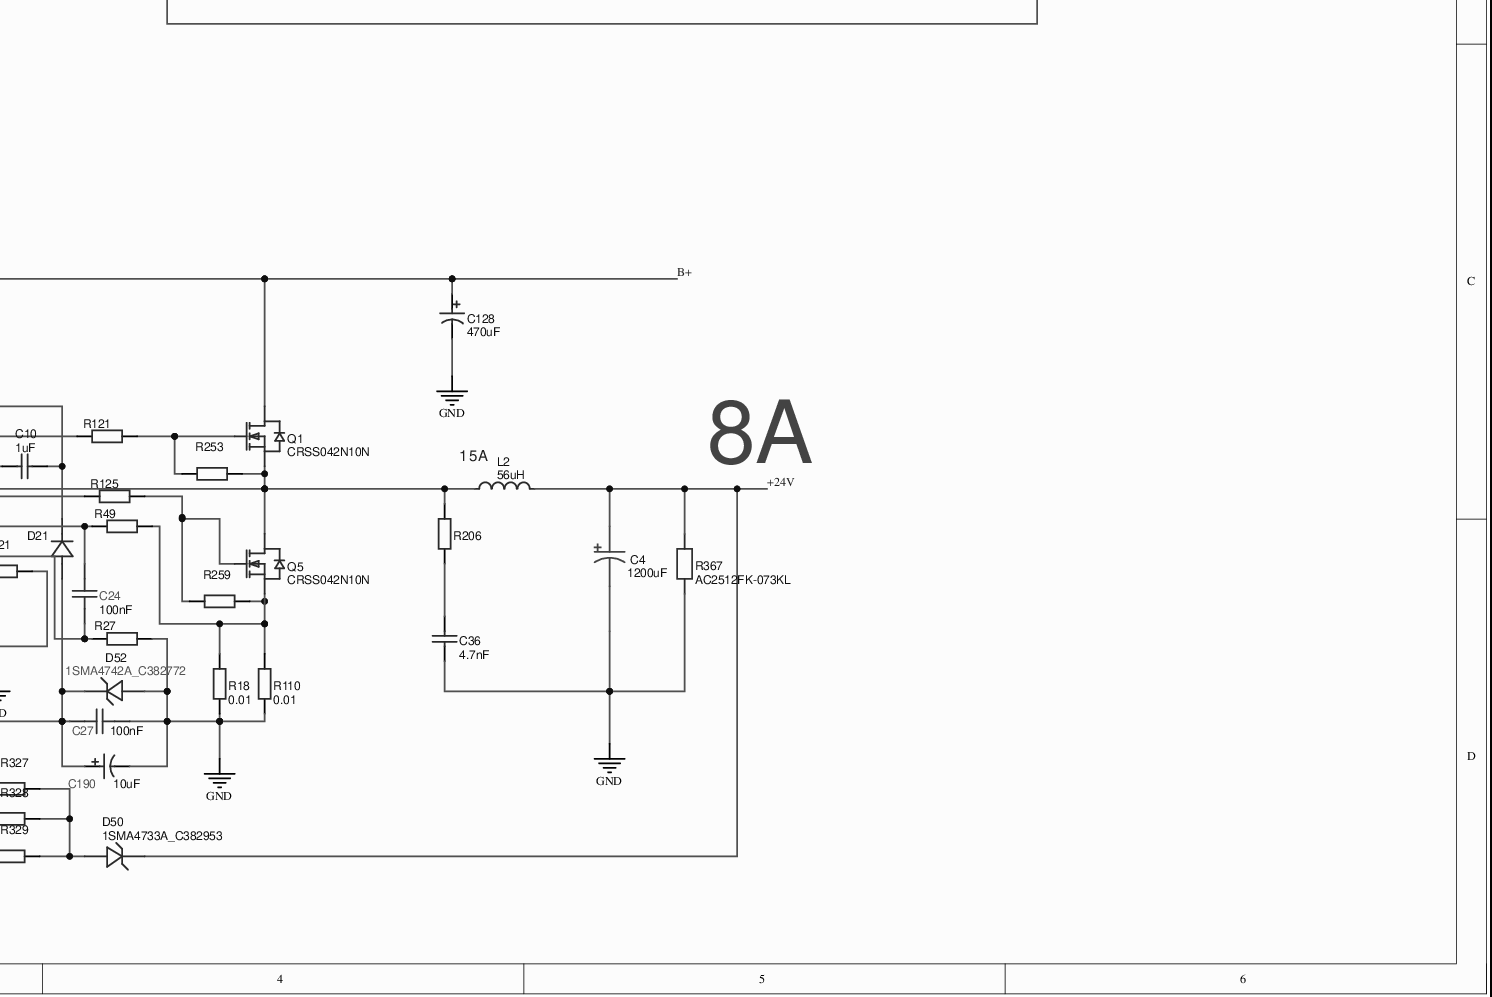
[diagram p0: MISC84402-12.SchDoc, bottom right]
# Altium project MISC84402-4.PrjPcb (part 5 of 7)
## Sheet MISC84402-12.SchDoc (continued)
### Library data of the parts (continued)
R34 = (no symbol name): BOM_Manufacturer: UniOhm; BOM_Manufacturer Part: 0603WAF7501T5E; nameAlias: Resistance; Resistance (Ohms): 7.5K; BOM_Supplier: LCSC; BOM_Supplier Part: C23234; BOM_JLCPCB Part Class: Basic Part; spicePre: R; spiceSymbolName: 0603WAF7501T5E
R48 R362 = (no symbol name): BOM_Manufacturer: UniOhm; BOM_Manufacturer Part: 0603WAF330JT5E; nameAlias: Resistance; Resistance (Ohms): 33; BOM_Supplier: LCSC; BOM_Supplier Part: C23140; BOM_JLCPCB Part Class: Basic Part; spicePre: R; spiceSymbolName: 0603WAF330JT5E
R51 R73 R291 R296 R302 R314 = 2K: BOM_Manufacturer: UniOhm; BOM_Manufacturer Part: 0603WAF2001T5E; nameAlias: Resistance (Ohms); BOM_Supplier: LCSC; BOM_Supplier Part: C22975; BOM_JLCPCB Part Class: Basic Part; spicePre: R; spiceSymbolName: 0603WAF2001T5E
R74 R101 R121 R125 = (no symbol name): BOM_Manufacturer: UniOhm; BOM_Manufacturer Part: 0805W8F220KT5E; nameAlias: Resistance; Resistance (Ohms): 2.2; BOM_Supplier: LCSC; BOM_Supplier Part: C17521; BOM_JLCPCB Part Class: Basic Part; spicePre: R; spiceSymbolName: 0805W8F220KT5E
R75 = (no symbol name): BOM_Manufacturer: UniOhm; BOM_Manufacturer Part: 0603WAF1003T5E; nameAlias: Resistance; Resistance (Ohms): 100K; BOM_Supplier: LCSC; BOM_Supplier Part: C25803; BOM_JLCPCB Part Class: Basic Part; spicePre: R; spiceSymbolName: 0603WAF1003T5E
R104 R297 R308 = 10K: BOM_Manufacturer: FH; BOM_Manufacturer Part: RS-03K102JT; nameAlias: Resistance (Ohms); BOM_Supplier: LCSC; BOM_Supplier Part: C73797; spicePre: R; spiceSymbolName: RS-03K102JT
R106 R108 R109 = (no symbol name): BOM_Manufacturer: Milliohm; BOM_Manufacturer Part: GX2512-2W-20mR-1%; Resistance (Ohms): 0.02; nameAlias: Resistance; Contributor: LCSC; BOM_Supplier: LCSC; BOM_Supplier Part: C500720; BOM_JLCPCB Part Class: Extended Part; spicePre: R; spiceSymbolName: GX2512-2W-20MR-1%
R112 R290 = (no symbol name): BOM_Manufacturer: UniOhm; BOM_Manufacturer Part: 0603WAF6802T5E; nameAlias: Resistance; Resistance (Ohms): 68K; BOM_Supplier: LCSC; BOM_Supplier Part: C23231; BOM_JLCPCB Part Class: Basic Part; spicePre: R; spiceSymbolName: 0603WAF6802T5E
R136 R253 R259-R261 = (no symbol name): BOM_Manufacturer: UniOhm; BOM_Manufacturer Part: 0603WAF3002T5E; nameAlias: Resistance; Resistance (Ohms): 30K; BOM_Supplier: LCSC; BOM_Supplier Part: C22984; BOM_JLCPCB Part Class: Basic Part; spicePre: R; spiceSymbolName: 0603WAF3002T5E
R142 R145 = (no symbol name): BOM_Manufacturer: UniOhm; BOM_Manufacturer Part: 0603WAF1004T5E; nameAlias: Resistance; Resistance (Ohms): 1M; BOM_Supplier: LCSC; BOM_Supplier Part: C22935; BOM_JLCPCB Part Class: Basic Part; spicePre: R; spiceSymbolName: 0603WAF1004T5E
R147 R271 R295 = 1K: BOM_Manufacturer: FH; BOM_Manufacturer Part: RS-03K102JT; nameAlias: Resistance (Ohms); BOM_Supplier: LCSC; BOM_Supplier Part: C73797; spicePre: R; spiceSymbolName: RS-03K102JT
R198 R206 = (no symbol name): BOM_Manufacturer: UniOhm; BOM_Manufacturer Part: 1206W4F220KT5E; nameAlias: Resistance; Resistance (Ohms): 2.2; BOM_Supplier: LCSC; BOM_Supplier Part: C17947; BOM_JLCPCB Part Class: Extended Part; spicePre: R; spiceSymbolName: 1206W4F220KT5E
R210 = (no symbol name): BOM_Manufacturer: UniOhm; BOM_Manufacturer Part: 0603WAF7500T5E; nameAlias: Resistance; Resistance (Ohms): 750; BOM_Supplier: LCSC; BOM_Supplier Part: C23241; BOM_JLCPCB Part Class: Basic Part; spicePre: R; spiceSymbolName: 0603WAF7500T5E
R248 = 36K: BOM_Manufacturer: KOA Speer Elec; BOM_Manufacturer Part: RK73B1JTTD363J; nameAlias: Resistance (Ohms); Contributor: LCSC; BOM_Supplier: LCSC; BOM_Supplier Part: C192548; BOM_JLCPCB Part Class: Extended Part; spicePre: R; spiceSymbolName: RK73B1JTTD363J
R326 = (no symbol name): BOM_Manufacturer: UniOhm; BOM_Manufacturer Part: 0603WAF220KT5E; nameAlias: Resistance; Resistance (Ohms): 2.2; BOM_Supplier: LCSC; BOM_Supplier Part: C22939; BOM_JLCPCB Part Class: Basic Part; spicePre: R; spiceSymbolName: 0603WAF220KT5E
R327-R329 = (no symbol name): BOM_Manufacturer: UniOhm; BOM_Manufacturer Part: 0805W8F8200T5E; nameAlias: Resistance; Resistance (Ohms): 820; BOM_Supplier: LCSC; BOM_Supplier Part: C17837; BOM_JLCPCB Part Class: Basic Part; spicePre: R; spiceSymbolName: 0805W8F8200T5E
R357 = (no symbol name): BOM_Manufacturer: UniOhm; BOM_Manufacturer Part: 0603WAF2203T5E; nameAlias: Resistance; Resistance (Ohms): 220K; BOM_Supplier: LCSC; BOM_Supplier Part: C22961; BOM_JLCPCB Part Class: Basic Part; spicePre: R; spiceSymbolName: 0603WAF2203T5E
R358 = (no symbol name): BOM_Manufacturer: UniOhm; BOM_Manufacturer Part: 25121WJ0301T4E; nameAlias: Resistance; Resistance (Ohms): 300; BOM_Supplier: LCSC; BOM_Supplier Part: C25482; BOM_JLCPCB Part Class: Extended Part; spicePre: R; spiceSymbolName: 25121WJ0301T4E
R367 = AC2512FK-073KL: BOM_Manufacturer: YAGEO; Contributor: LCSC; BOM_Supplier: LCSC; BOM_Supplier Part: C728188; BOM_Manufacturer Part: AC2512FK-073KL; BOM_JLCPCB Part Class: Extended Part; spicePre: R; spiceSymbolName: AC2512FK-073KL
U1 U3 = LM5116MHX: BOM_Manufacturer: TI; BOM_Supplier: LCSC; BOM_Manufacturer Part: LM5116MHX; BOM_Supplier Part: C13755; BOM_JLCPCB Part Class: Extended Part; spicePre: U; spiceSymbolName: LM5116MHX
U2 = EG358: BOM_Manufacturer: EG; BOM_Supplier: LCSC; BOM_Manufacturer Part: EG358; BOM_Supplier Part: C111033; BOM_JLCPCB Part Class: Extended Part; spicePre: U; spiceSymbolName: EG358

## Sheet MISC84402-5.SchDoc
size 461 x 325 mm
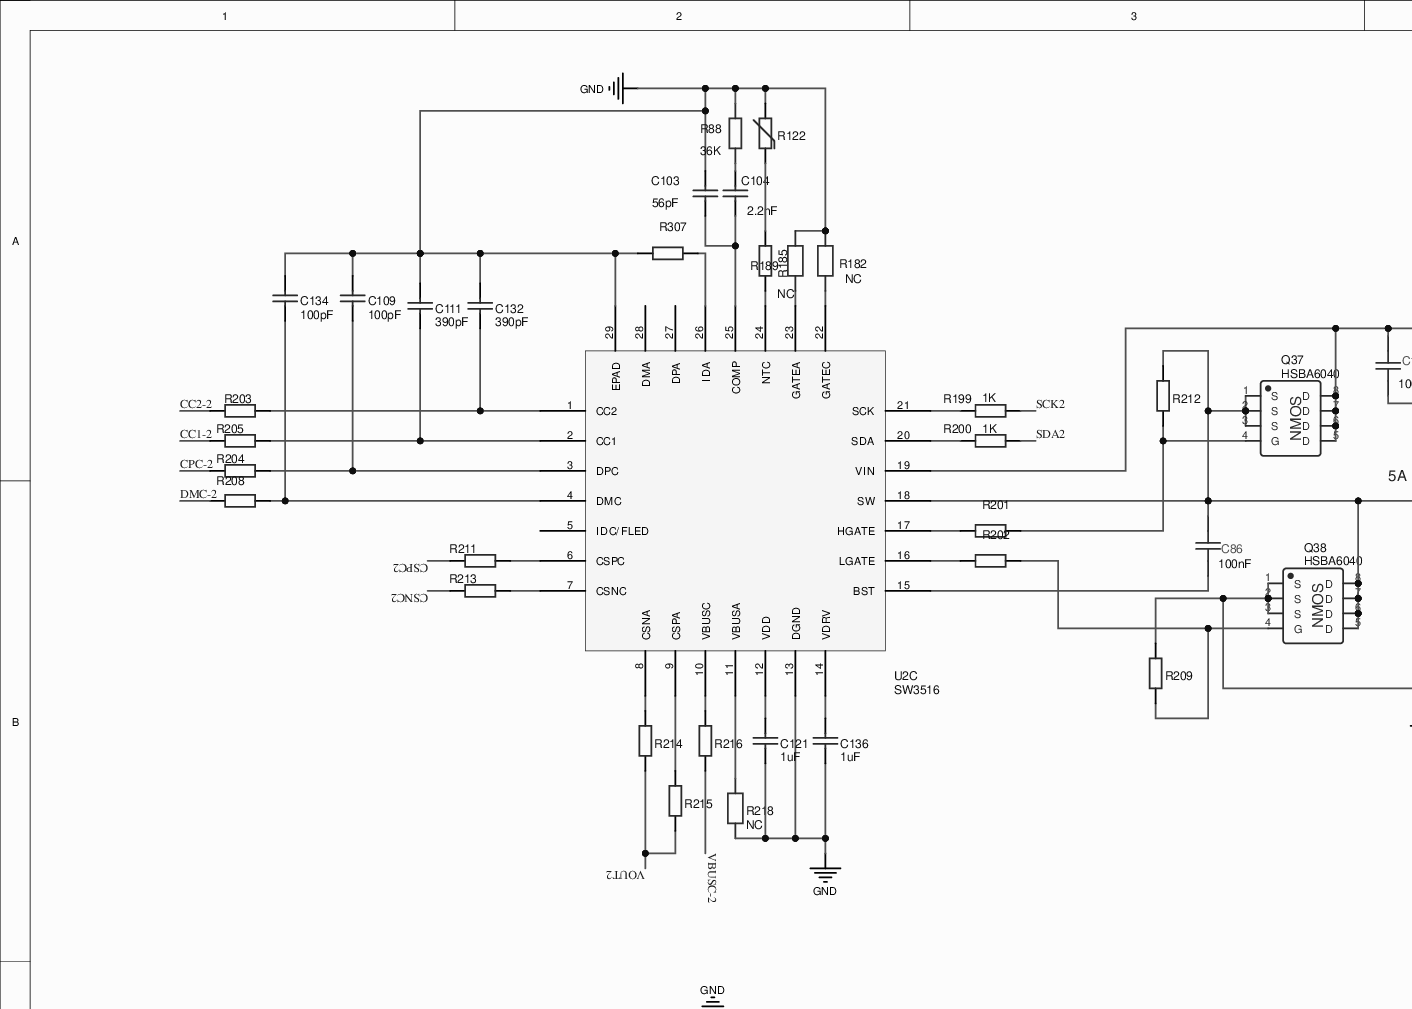
[diagram p1: MISC84402-5.SchDoc, top left]
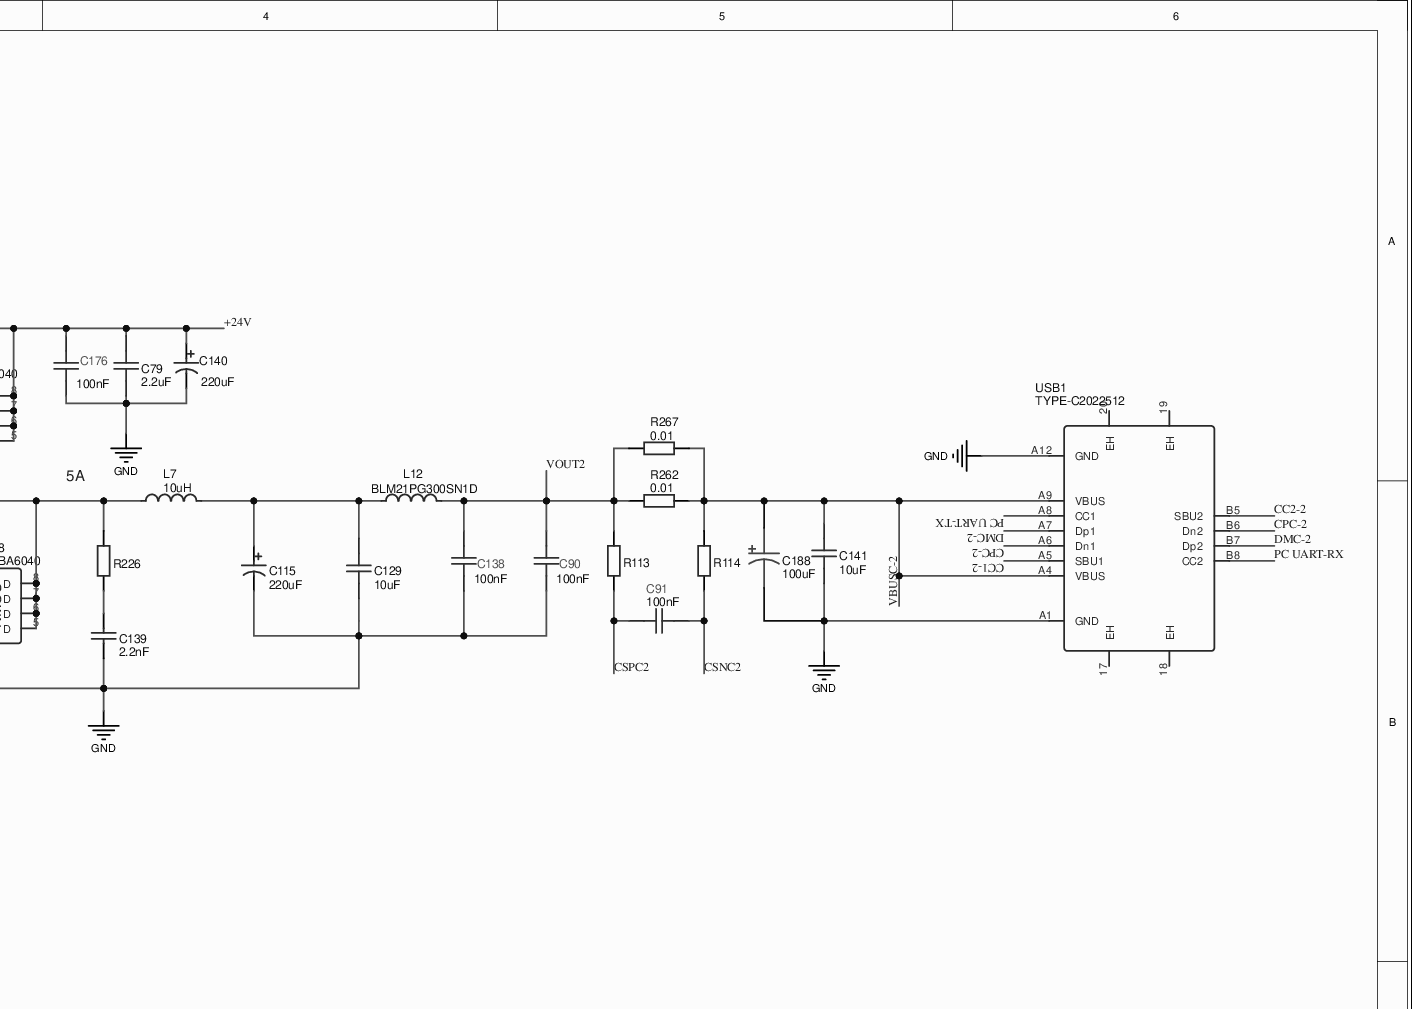
[diagram p2: MISC84402-5.SchDoc, top right]
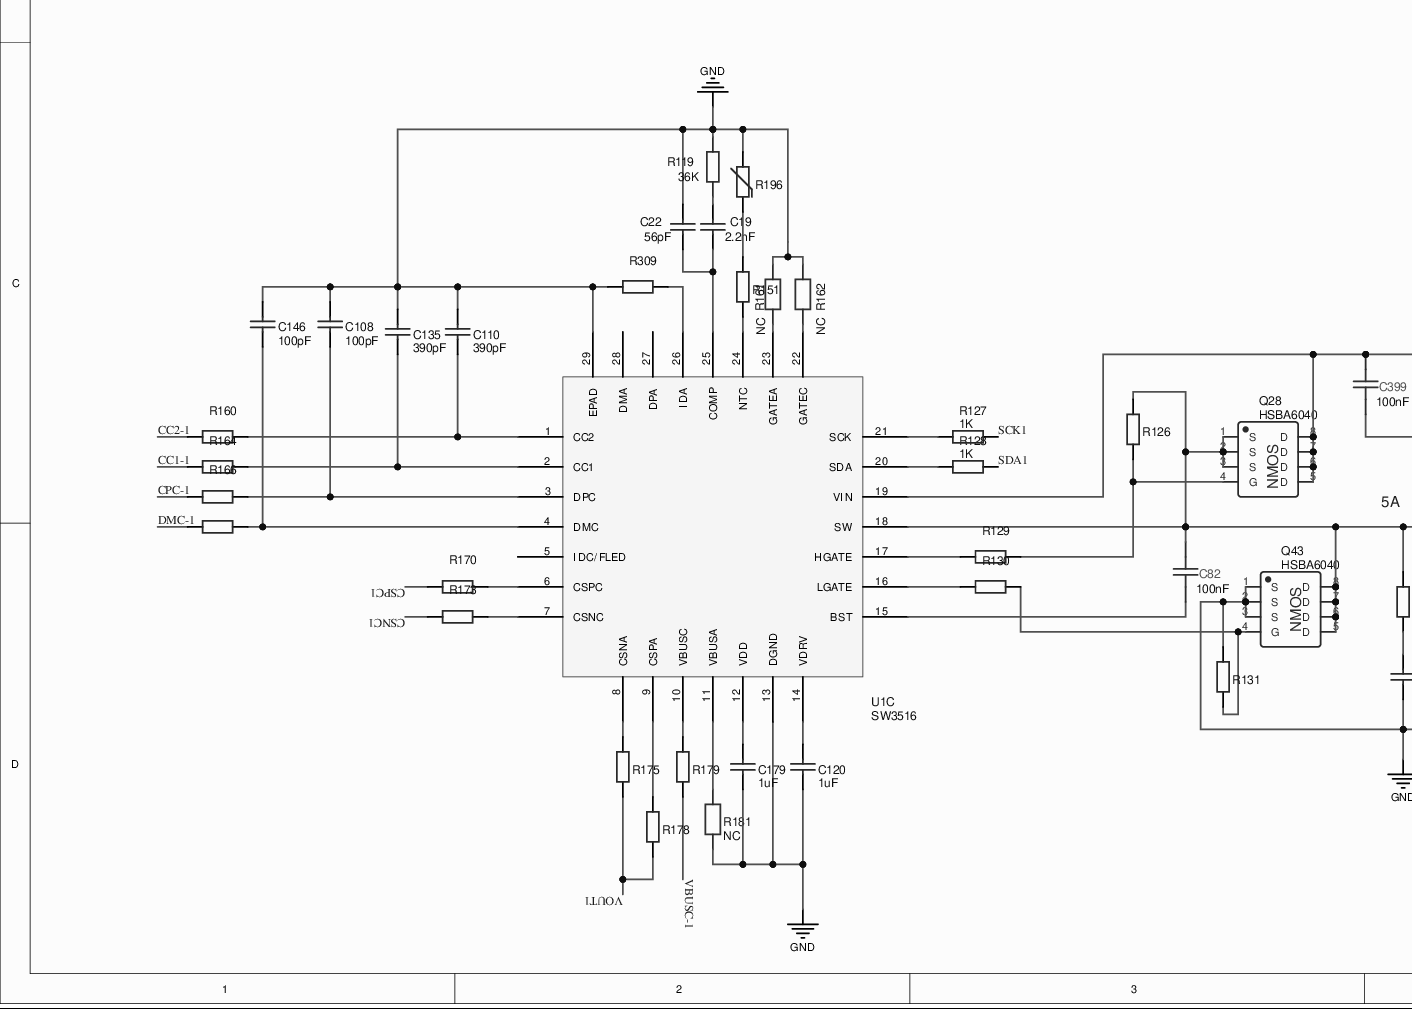
[diagram p3: MISC84402-5.SchDoc, bottom left]
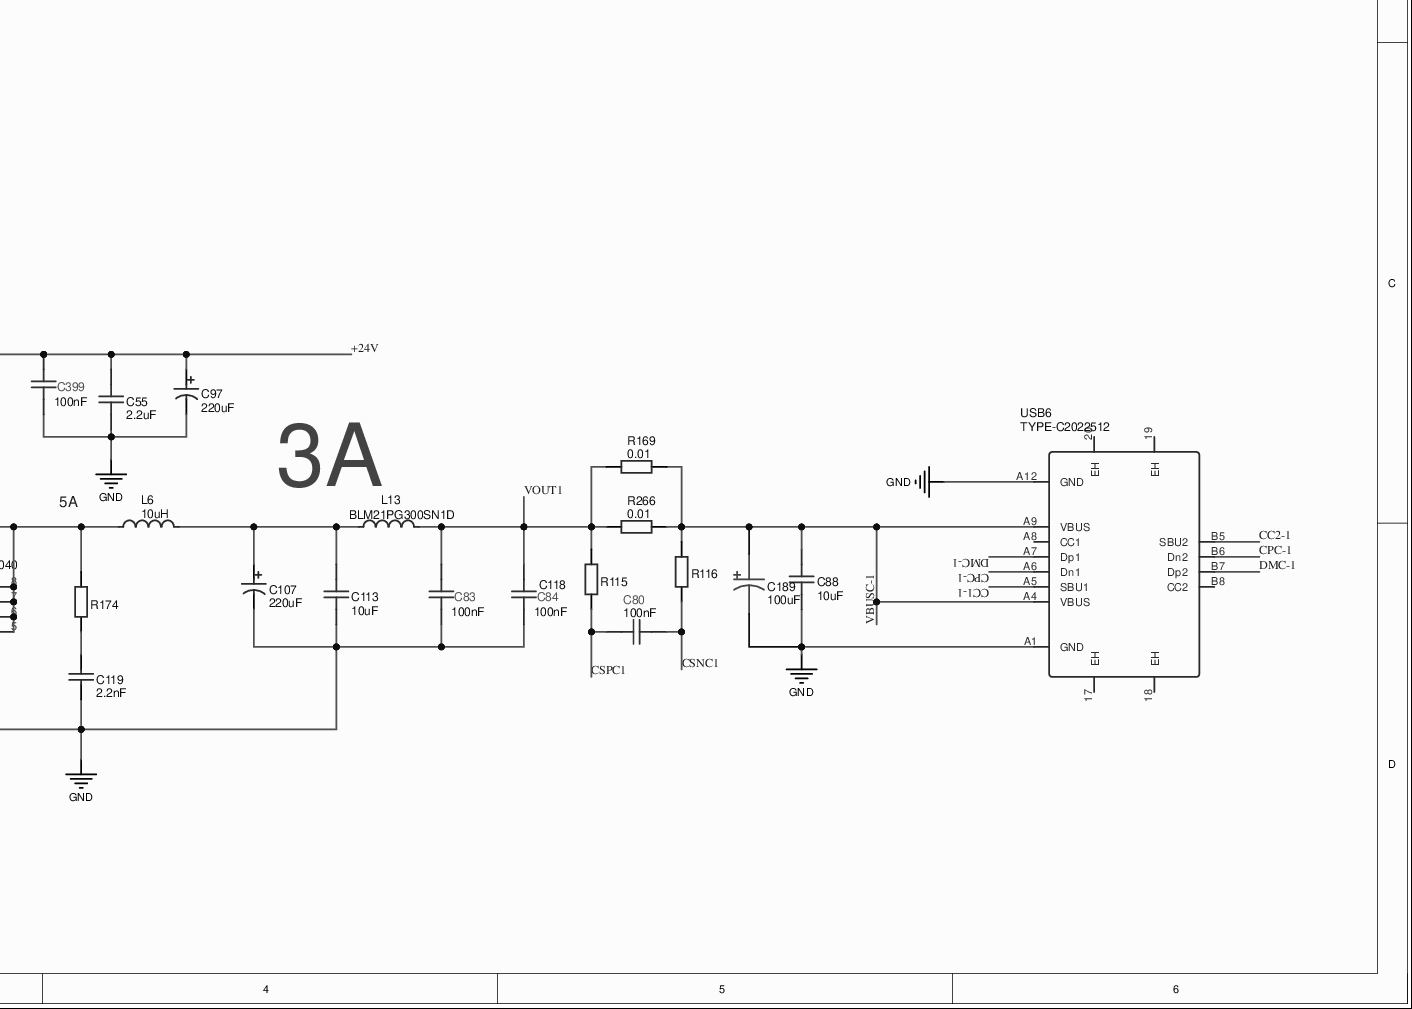
[diagram p4: MISC84402-5.SchDoc, bottom right]

### Parts
C19  2.2nF  [C0603]
C22  56pF  [C0603]
C55  2.2uF  [C0603]
C79  2.2uF  [C0603]
C80  100nF  [C0603]
C82  100nF  [C0603]
C83  100nF  [C0603]
C84  100nF  [C0603]
C86  100nF  [C0603]
C88  10uF  [C0603]
C90  100nF  [C0603]
C91  100nF  [C0603]
C97  220uF  [CAP-TH_BD8.0-P3.50-D0.6-FD]
C103  56pF  [C0603]
C104  2.2nF  [C0603]
C107  220uF  [CAP-TH_BD8.0-P3.50-D0.6-FD]
C108  100pF  [C0603]
C109  100pF  [C0603]
C110  390pF  [C0603]
C111  390pF  [C0603]
C113  10uF  [C0603]
C115  220uF  [CAP-TH_BD8.0-P3.50-D0.6-FD]
C119  2.2nF  [C0603]
C120  1uF  [C0603]
C121  1uF  [C0603]
C129  10uF  [C0603]
C132  390pF  [C0603]
C134  100pF  [C0603]
C135  390pF  [C0603]
C136  1uF  [C0603]
C138  100nF  [C0603]
C139  2.2nF  [C0603]
C140  220uF  [CAP-TH_BD8.0-P3.50-D0.6-FD]
C141  10uF  [C0603]
C146  100pF  [C0603]
C176  100nF  [C0603]
C179  1uF  [C0603]
C188  100uF  [CAP-TH_BD6.3-P2.50-D1.0-FD]
C189  100uF  [CAP-TH_BD6.3-P2.50-D1.0-FD]
C399  100nF  [C0603]
L6  10uH  [IND-SMD_L13.8-W12.6_YSPI13XX]
L7  10uH  [IND-SMD_L13.8-W12.6_YSPI13XX]
L12  BLM21PG300SN1D  [L0805]
L13  BLM21PG300SN1D  [L0805]
Q28  HSBA6040  [POWERPAK-SO-8_L6.2-W5.2-P1.27-BR-EP]
Q37  HSBA6040  [POWERPAK-SO-8_L6.2-W5.2-P1.27-BR-EP]
Q38  HSBA6040  [POWERPAK-SO-8_L6.2-W5.2-P1.27-BR-EP]
Q43  HSBA6040  [POWERPAK-SO-8_L6.2-W5.2-P1.27-BR-EP]
R88  36K  [R0603]
R113  (no value)  [R0603]
R114  (no value)  [R0603]
R115  (no value)  [R0603]
R116  (no value)  [R0603]
R119  36K  [R0603]
R122  (no value)  [R0603]
R126  (no value)  [R0603]
R127  1K  [R0603]
R128  1K  [R0603]
R129  (no value)  [R0603]
R130  (no value)  [R0603]
R131  (no value)  [R0603]
R151  (no value)  [R0603]
R160  (no value)  [R0603]
R161  NC  [R0603]
R162  NC  [R0603]
R164  (no value)  [R0603]
R166  (no value)  [R0603]
R167  (no value)  [R0603]
R169  0.01  [R2512]
R170  (no value)  [R0603]
R173  (no value)  [R0603]
R174  (no value)  [R0603]
R175  (no value)  [R0603]
R178  (no value)  [R0603]
R179  (no value)  [R0603]
R181  NC  [R0603]
R182  NC  [R0603]
R185  NC  [R0603]
R189  (no value)  [R0603]
R196  (no value)  [R0603]
R199  1K  [R0603]
R200  1K  [R0603]
R201  (no value)  [R0603]
R202  (no value)  [R0603]
R203  (no value)  [R0603]
R204  (no value)  [R0603]
R205  (no value)  [R0603]
R208  (no value)  [R0603]
R209  (no value)  [R0603]
R211  (no value)  [R0603]
R212  (no value)  [R0603]
R213  (no value)  [R0603]
R214  (no value)  [R0603]
R215  (no value)  [R0603]
R216  (no value)  [R0603]
R218  NC  [R0603]
R226  (no value)  [R0603]
R262  0.01  [R2512]
R266  0.01  [R2512]
R267  0.01  [R2512]
R307  (no value)  [R0603]
R309  (no value)  [R0603]
U1C  (no value)  [QFN-28_L4.0-W4.0-P0.40-BL-EP]
U2C  (no value)  [QFN-28_L4.0-W4.0-P0.40-BL-EP]
USB1  TYPE-C2022512  [NEW_TYPEC]
USB6  TYPE-C2022512  [NEW_TYPEC]

### Nets
GND: C22.2 C55.1 C79.1 C83.1 C84.1 C88.1 C90.1 C97.2 C103.1 C107.2 C108.2 C109.2 C110.2 C111.2 C113.1 C115.2 C119.1 C120.1 C121.1 C129.1 C132.2 C134.2 C135.2 C136.1 C138.1 C139.1 C140.2 C141.1 C146.2 C176.1 C179.1 C188.2 C189.2 C399.1 Q38.1(S) Q38.2(S) Q38.3(S) Q43.1(S) Q43.2(S) Q43.3(S) R88.2 R119.2 R122.2 R131.2 R161.2 R162.2 R181.2 R182.2 R185.2 R196.2 R209.2 R218.2 R307.1 R309.1 U1C.13(DGND) U1C.29(EPAD) U2C.13(DGND) U2C.29(EPAD) USB1.A1(GND) USB1.A12(GND) USB6.A1(GND) USB6.A12(GND)
+24V: C55.2 C79.2 C97.1 C140.1 C176.2 C399.2 Q28.5(D) Q28.6(D) Q28.7(D) Q28.8(D) Q37.5(D) Q37.6(D) Q37.7(D) Q37.8(D) U1C.19(VIN) U2C.19(VIN)
CC1-1: R164.1 USB6.A5(SBU1)
CC1-2: R205.1 USB1.A5(SBU1)
CC2-1: R160.1 USB6.B5(SBU2)
CC2-2: R203.1 USB1.B5(SBU2)
CPC-1: R166.1 USB6.A6(Dn1) USB6.B6(Dn2)
CPC-2: R204.1 USB1.A6(Dn1) USB1.B6(Dn2)
CSNC1: C80.1 R116.1 R173.1
CSNC2: C91.1 R114.1 R213.1
CSPC1: C80.2 R115.1 R170.1
CSPC2: C91.2 R113.1 R211.1
DMC-1: R167.1 USB6.A7(Dp1) USB6.B7(Dp2)
DMC-2: R208.1 USB1.A7(Dp1) USB1.B7(Dp2)
PC UART-RX: USB1.B8(CC2)
PC UART-TX: USB1.A8(CC1)
SCK1: R127.2
SCK2: R199.2
SDA1: R128.2
SDA2: R200.2
VBUSC-1: C88.2 C189.1 R116.2 R169.2 R179.1 R266.2 USB6.A4(VBUS) USB6.A9(VBUS)
VBUSC-2: C141.2 C188.1 R114.2 R216.1 R262.2 R267.2 USB1.A4(VBUS) USB1.A9(VBUS)
VOUT1: C83.2 C84.2 L13.2 R115.2 R169.1 R175.1 R178.1 R266.1
VOUT2: C90.2 C138.2 L12.2 R113.2 R214.1 R215.1 R262.1 R267.1
NetC19_1: C19.1 C22.1 U1C.25(COMP)
NetC19_2: C19.2 R119.1
NetC82_1: C82.1 U1C.15(BST)
NetC82_2: C82.2 L6.1(S) Q28.1(S) Q28.2(S) Q28.3(S) Q43.5(D) Q43.6(D) Q43.7(D) Q43.8(D) R126.2 R174.2 U1C.18(SW)
NetC86_1: C86.1 U2C.15(BST)
NetC86_2: C86.2 L7.1(S) Q37.1(S) Q37.2(S) Q37.3(S) Q38.5(D) Q38.6(D) Q38.7(D) Q38.8(D) R212.2 R226.2 U2C.18(SW)
NetC103_2: C103.2 C104.1 U2C.25(COMP)
NetC104_2: C104.2 R88.1
NetC107_1: C107.1 C113.2 L6.2(F) L13.1
NetC108_1: C108.1 R166.2 U1C.3(DPC)
NetC109_1: C109.1 R204.2 U2C.3(DPC)
NetC110_1: C110.1 R160.2 U1C.1(CC2)
NetC111_1: C111.1 R205.2 U2C.2(CC1)
NetC115_1: C115.1 C129.2 L7.2(F) L12.1
NetC119_2: C119.2 R174.1
NetC120_2: C120.2 U1C.14(VDRV)
NetC121_2: C121.2 U2C.12(VDD)
NetC132_1: C132.1 R203.2 U2C.1(CC2)
NetC134_1: C134.1 R208.2 U2C.4(DMC)
NetC135_1: C135.1 R164.2 U1C.2(CC1)
NetC136_2: C136.2 U2C.14(VDRV)
NetC139_2: C139.2 R226.1
NetC146_1: C146.1 R167.2 U1C.4(DMC)
NetC179_2: C179.2 U1C.12(VDD)
NetQ28_4: Q28.4(G) R126.1 R129.2
NetQ37_4: Q37.4(G) R201.2 R212.1
NetQ38_4: Q38.4(G) R202.2 R209.1
NetQ43_4: Q43.4(G) R130.2 R131.1
NetR122_1: R122.1 R189.2
NetR127_1: R127.1 U1C.21(SCK)
NetR128_1: R128.1 U1C.20(SDA)
NetR129_1: R129.1 U1C.17(HGATE)
NetR130_1: R130.1 U1C.16(LGATE)
NetR151_1: R151.1 U1C.24(NTC)
NetR151_2: R151.2 R196.1
NetR161_1: R161.1 U1C.23(GATEA)
NetR162_1: R162.1 U1C.22(GATEC)
NetR170_2: R170.2 U1C.6(CSPC)
NetR173_2: R173.2 U1C.7(CSNC)
NetR175_2: R175.2 U1C.8(CSNA)
NetR178_2: R178.2 U1C.9(CSPA)
NetR179_2: R179.2 U1C.10(VBUSC)
NetR181_1: R181.1 U1C.11(VBUSA)
NetR182_1: R182.1 U2C.22(GATEC)
NetR185_1: R185.1 U2C.23(GATEA)
NetR189_1: R189.1 U2C.24(NTC)
NetR199_1: R199.1 U2C.21(SCK)
NetR200_1: R200.1 U2C.20(SDA)
NetR201_1: R201.1 U2C.17(HGATE)
NetR202_1: R202.1 U2C.16(LGATE)
NetR211_2: R211.2 U2C.6(CSPC)
NetR213_2: R213.2 U2C.7(CSNC)
NetR214_2: R214.2 U2C.8(CSNA)
NetR215_2: R215.2 U2C.9(CSPA)
NetR216_2: R216.2 U2C.10(VBUSC)
NetR218_1: R218.1 U2C.11(VBUSA)
NetR307_2: R307.2 U2C.26(IDA)
NetR309_2: R309.2 U1C.26(IDA)

Not connected (* = marked no-connect by the designer): U1C 5(IDC/FLED) 27(DPA) 28(DMA); U2C 5(IDC/FLED) 27(DPA) 28(DMA); USB1 17(EH) 18(EH) 19(EH) 20(EH); USB6 17(EH) 18(EH) 19(EH) 20(EH) A8(CC1) B8(CC2)

### Notes on the sheet
- 5A
- (near L13) 3A
- (near C84) C118

### Library data of the parts
C19 C104 = 2.2nF: as C20 on sheet MISC84402-12; BOM_Supplier: LCSC; BOM_Supplier Part: C16033; BOM_JLCPCB Part Class: Extended Part; spicePre: C; spiceSymbolName: CL10B222KB8NNNC
C22 C103 = 56pF: as C18 on sheet MISC84402-12; BOM_Supplier: LCSC; BOM_Supplier Part: C39148; BOM_JLCPCB Part Class: Basic Part; spicePre: C; spiceSymbolName: CL10C560JB8NNNC
C55 C79 = 2.2uF: BOM_Manufacturer Part: CL10A225KB8NNNC; Contributor: LCSC; nameAlias: Capacitance; BOM_Supplier: LCSC; BOM_Supplier Part: C913904; BOM_JLCPCB Part Class: Extended Part; spicePre: C; spiceSymbolName: CL10A225KB8NNNC
C80 C82-C84 C86 C90 C91 C138 C176 C399 = 100nF: as C1 on sheet MISC84402-12; BOM_Supplier: LCSC; BOM_Supplier Part: C15725; BOM_JLCPCB Part Class: Extended Part; spicePre: C; spiceSymbolName: CL10B104KC8NNNC
C88 C113 C129 C141 = 10uF: BOM_Manufacturer: FH(Guangdong Fenghua Advanced Tech); BOM_Manufacturer Part: 0603X106M250NT; nameAlias: Capacitance; Contributor: LCSC; BOM_Supplier: LCSC; BOM_Supplier Part: C479655; BOM_JLCPCB Part Class: Extended Part; spicePre: C; spiceSymbolName: 0603X106M250NT
C97 C107 C115 C140 = 220uF: BOM_Manufacturer: Rubycon; BOM_Manufacturer Part: 35ZLH220MEFC8X11.5; nameAlias: Capacitance; BOM_Supplier: LCSC; BOM_Supplier Part: C107639; BOM_JLCPCB Part Class: Extended Part; spicePre: C; spiceSymbolName: 35ZLH220MEFC8X11.5
C108 C109 C134 C146 = 100pF: BOM_Manufacturer Part: CL10C101JB8NNNC; BOM_Manufacturer: SAMSUNG; nameAlias: Capacitance; BOM_Supplier: LCSC; BOM_Supplier Part: C14858; BOM_JLCPCB Part Class: Basic Part; spicePre: C; spiceSymbolName: CL10C101JB8NNNC
C110 C111 C132 C135 = 390pF: BOM_Manufacturer: FH; BOM_Manufacturer Part: 0603B391K500NT; nameAlias: Capacitance; BOM_Supplier: LCSC; BOM_Supplier Part: C1617; BOM_JLCPCB Part Class: Extended Part; spicePre: C; spiceSymbolName: 0603B391K500NT
C119 C139 = 2.2nF: BOM_Manufacturer: FH; BOM_Manufacturer Part: 0603B222K500NT; nameAlias: Capacitance; BOM_Supplier: LCSC; BOM_Supplier Part: C1604; BOM_JLCPCB Part Class: Basic Part; spicePre: C; spiceSymbolName: 0603B222K500NT
C120 C121 C136 C179 = 1uF: as C10 on sheet MISC84402-12; BOM_Supplier: LCSC; BOM_Supplier Part: C15849; BOM_JLCPCB Part Class: Basic Part; spicePre: C; spiceSymbolName: CL10A105KB8NNNC
C188 C189 = 100uF: BOM_Manufacturer: Rubycon; BOM_Manufacturer Part: 25YXF100MFFC6.3X11; nameAlias: Capacitance; Contributor: LCSC; BOM_Supplier: LCSC; BOM_Supplier Part: C125770; BOM_JLCPCB Part Class: Extended Part; spicePre: C; spiceSymbolName: 25YXF100MFFC6.3X11
L6 L7 = 10uH: BOM_Manufacturer: Bao Cheng Elec; BOM_Manufacturer Part: BCIHP1350-6R8M; nameAlias: Inductance; Contributor: LCSC; BOM_Supplier: LCSC; BOM_Supplier Part: C237964; BOM_JLCPCB Part Class: Extended Part; spicePre: L; spiceSymbolName: BCIHP1350-6R8M
L12 L13 = BLM21PG300SN1D: BOM_Manufacturer: MuRata; nameAlias: Value(H); BOM_Supplier: LCSC; BOM_Manufacturer Part: BLM21PG300SN1D; BOM_Supplier Part: C16903; BOM_JLCPCB Part Class: Extended Part; spicePre: L; spiceSymbolName: BLM21PG300SN1D
Q28 Q37 Q38 Q43 = HSBA6040: BOM_Manufacturer: HUASHUO; Contributor: LCSC; BOM_Supplier: LCSC; BOM_Supplier Part: C508831; BOM_Manufacturer Part: HSBA6040; BOM_JLCPCB Part Class: Extended Part; spicePre: Q; spiceSymbolName: HSBA6040
R88 R119 = 36K: as R248 on sheet MISC84402-12; BOM_Supplier: LCSC; BOM_Supplier Part: C192548; BOM_JLCPCB Part Class: Extended Part; spicePre: R; spiceSymbolName: RK73B1JTTD363J
R113-R116 R174 R226 = (no symbol name): as R22 on sheet MISC84402-12; BOM_Supplier: LCSC; BOM_Supplier Part: C22936; BOM_JLCPCB Part Class: Basic Part; spicePre: R; spiceSymbolName: 0603WAF100KT5E
R122 R196 = (no symbol name): BOM_Manufacturer: MuRata; BOM_Manufacturer Part: NCP18XH103F03RB; nameAlias: Value; BOM_Supplier: LCSC; BOM_Supplier Part: C13564; BOM_JLCPCB Part Class: Extended Part; spicePre: R; spiceSymbolName: NCP18XH103F03RB
R126 R131 R209 R212 = (no symbol name): as R136 on sheet MISC84402-12; BOM_Supplier: LCSC; BOM_Supplier Part: C22984; BOM_JLCPCB Part Class: Basic Part; spicePre: R; spiceSymbolName: 0603WAF3002T5E
R127 R128 R199 R200 = 1K: as R147 on sheet MISC84402-12; BOM_Supplier: LCSC; BOM_Supplier Part: C73797; spicePre: R; spiceSymbolName: RS-03K102JT
R129 R130 R201 R202 = (no symbol name): as R326 on sheet MISC84402-12; BOM_Supplier: LCSC; BOM_Supplier Part: C22939; BOM_JLCPCB Part Class: Basic Part; spicePre: R; spiceSymbolName: 0603WAF220KT5E
R151 R189 = (no symbol name): as R14 on sheet MISC84402-12; BOM_Supplier: LCSC; BOM_Supplier Part: C22975; BOM_JLCPCB Part Class: Basic Part; spicePre: R; spiceSymbolName: 0603WAF2001T5E
R160 R164 R166 R167 R170 R173 R175 R178 R179 R203-R205 R208 R211 R213-R216 R307 R309 = (no symbol name): as R15 on sheet MISC84402-12; BOM_Supplier: LCSC; BOM_Supplier Part: C21189; BOM_JLCPCB Part Class: Basic Part; spicePre: R; spiceSymbolName: 0603WAF0000T5E
R161 R162 R181 R182 R185 R218 = NC: Contributor: LCEDA_Lib; spicePre: R
  R161 R162 R182 R185: spiceSymbolName: R_0805_EU
  R181 R218: spiceSymbolName: R_0603_EU
R169 R262 R266 R267 = 0.01: as R18 on sheet MISC84402-12; BOM_Supplier Part: C76272; BOM_Supplier: LCSC; BOM_JLCPCB Part Class: Extended Part; spicePre: R; spiceSymbolName: MRF6432(2512)LR010JTS
U1C U2C = SW3516: Part Number: E02P00432; MPN: SW3516H; Power: 6~40V; Component: Standard; Contributor: dcy2237; Footprint: QFN28_4X4_EPAD; Availability: A; ComponentLink1Description: Datasheet; spicePre: U; spiceSymbolName: SW3516; Comment_1: SW3516
USB1 USB6 = TYPE-C2022512: BOM_Manufacturer Part: TYPE-C-31-D-09; Contributor: z123tt; BOM_Supplier: LCSC; BOM_Supplier Part: C2848615; BOM_JLCPCB Part Class: Extended Part; spicePre: U; spiceSymbolName: TYPE-C2022512